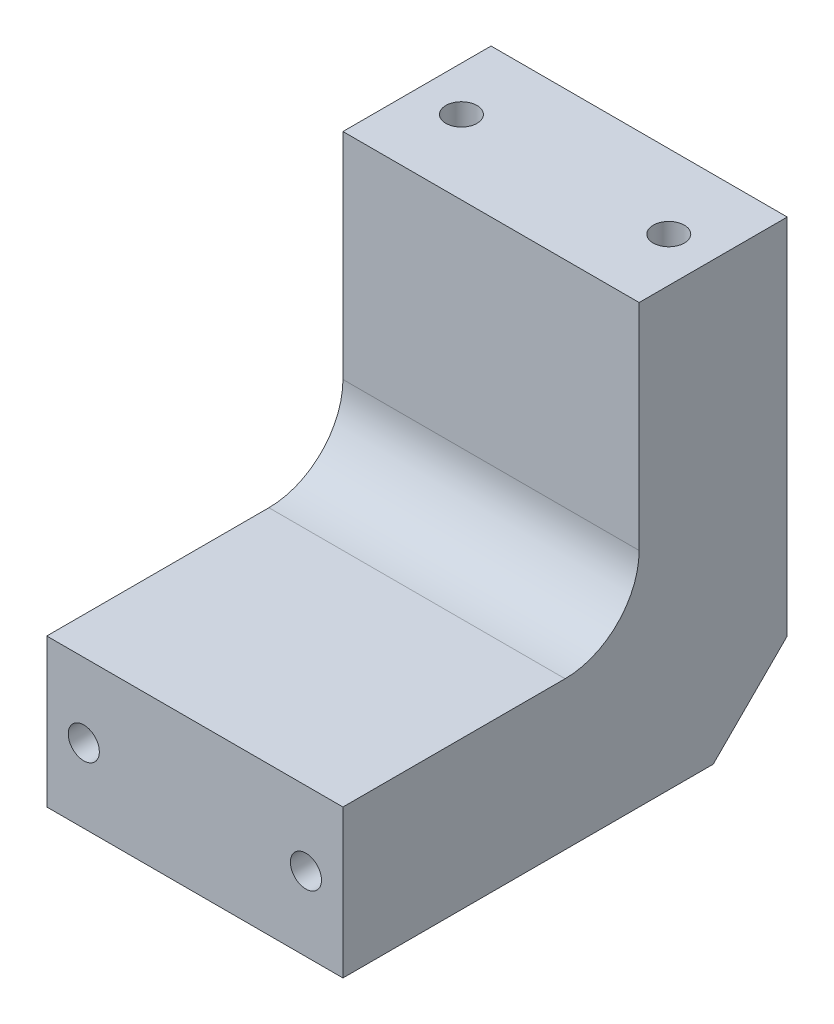
from build123d import *

# Parameters (mm, degrees)
SKETCH1_W             = 40
SKETCH1_H             = 60
BOSS_EXTRUDE1_DEPTH   = 59
SKETCH2_W             = 40
SKETCH2_H             = 39
CUT_EXTRUDE1_DEPTH    = 45
CHAMFER1_SIZE         = 10
FILLET1_R             = 10
M5_TAPPED_HOLE1_D     = 4.2
M5_TAPPED_HOLE1_DEPTH = 12.4
M5_TAPPED_HOLE1_TIP   = 1.2618073
M5_TAPPED_HOLE2_D     = 4.2
M5_TAPPED_HOLE2_DEPTH = 12.4
M5_TAPPED_HOLE2_TIP   = 1.2618073


with BuildPart() as part:
    # Sketch1 → Boss-Extrude1 (new body)
    with BuildSketch(Plane(origin=(0, 0, 0), x_dir=(1, 0, 0), z_dir=(0, 1, 0))):
        Rectangle(SKETCH1_W, SKETCH1_H)
    extrude(amount=BOSS_EXTRUDE1_DEPTH)

    # Sketch2 → Cut-Extrude1 (cut)
    with BuildSketch(Plane(origin=(20, 0, 0), x_dir=(0, 0, -1), z_dir=(1, 0, 0))):
        with Locations((-10, 39.5)):
            Rectangle(SKETCH2_W, SKETCH2_H)
    extrude(amount=-CUT_EXTRUDE1_DEPTH, mode=Mode.SUBTRACT)

    # Chamfer1
    chamfer1_edges = [part.edges().sort_by_distance(p)[0] for p in [
        (0, 0, -30),
    ]]
    chamfer(chamfer1_edges, length=CHAMFER1_SIZE)

    # Fillet1
    fillet1_edges = [part.edges().sort_by_distance(p)[0] for p in [
        (0, 20, -10),
    ]]
    fillet(fillet1_edges, radius=FILLET1_R)

    # M5 Tapped Hole1
    with Locations(Plane(origin=(-14, 59, -20), x_dir=(0, 0, 1), z_dir=(0, 1, 0))):
        with Locations((0, 0), (0, 28)):
            Hole(M5_TAPPED_HOLE1_D / 2, depth=M5_TAPPED_HOLE1_DEPTH)
            with Locations((0, 0, -(M5_TAPPED_HOLE1_DEPTH + M5_TAPPED_HOLE1_TIP / 2))):  # 118° drill point
                Cone(0, M5_TAPPED_HOLE1_D / 2, M5_TAPPED_HOLE1_TIP, mode=Mode.SUBTRACT)

    # M5 Tapped Hole2
    with Locations(Plane(origin=(-15, 10, 30), x_dir=(1, 0, 0), z_dir=(0, 0, 1))):
        with Locations((0, 0), (30, 0)):
            Hole(M5_TAPPED_HOLE2_D / 2, depth=M5_TAPPED_HOLE2_DEPTH)
            with Locations((0, 0, -(M5_TAPPED_HOLE2_DEPTH + M5_TAPPED_HOLE2_TIP / 2))):  # 118° drill point
                Cone(0, M5_TAPPED_HOLE2_D / 2, M5_TAPPED_HOLE2_TIP, mode=Mode.SUBTRACT)


solid = part.part
